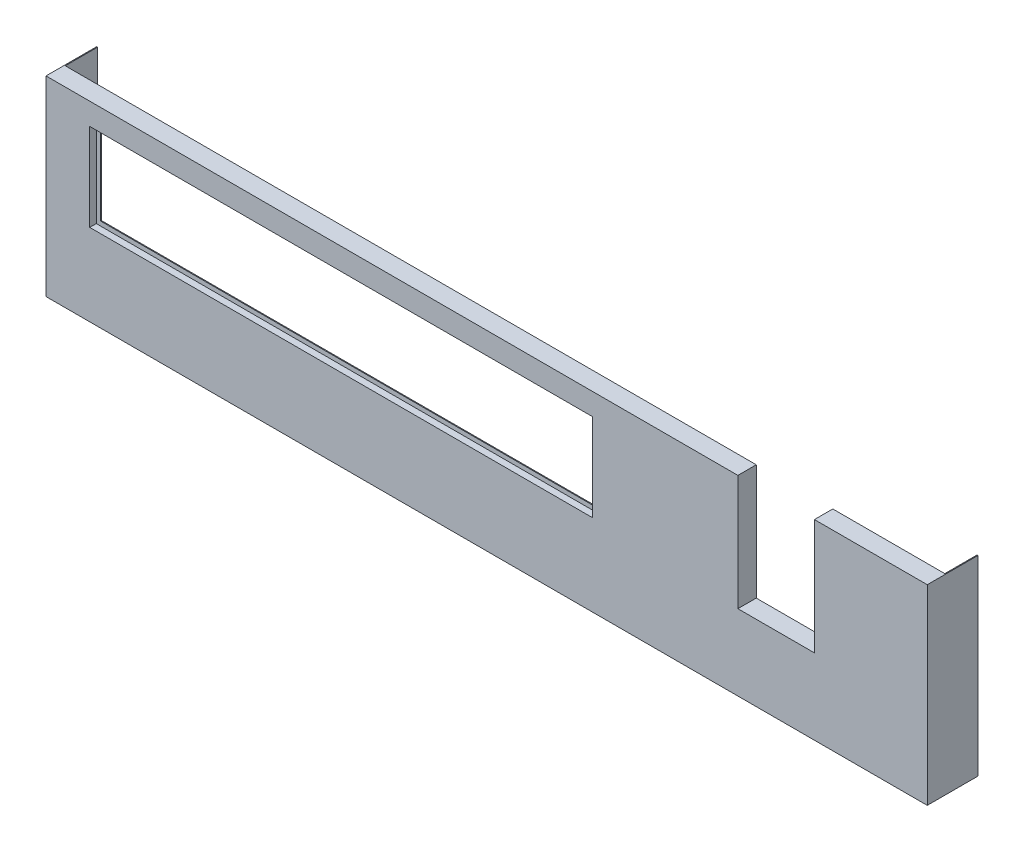
from build123d import *

# Parameters (mm, degrees)
EXTRUDE_1_DEPTH     = 2
SKETCH_7_W          = 2
SKETCH_7_H          = 437
EXTRUDE_2_DEPTH     = 114
SKETCH_8_W          = 2
SKETCH_8_H          = 437
EXTRUDE_3_DEPTH     = 114
EXTRUDE_4_DEPTH     = 40
SKETCH_10_W         = 1150
SKETCH_10_H         = 200
CUT_EXTRUDE_1_DEPTH = 10
SKETCH_11_W         = 2015
SKETCH_11_H         = 42.467862918
EXTRUDE_5_DEPTH     = 2
SKETCH_12_W         = 1154
SKETCH_12_H         = 204
SKETCH_12_W_2       = 1150
SKETCH_12_H_2       = 200
EXTRUDE_6_DEPTH     = 15
SKETCH_13_W         = 1154
SKETCH_13_H         = 204
SKETCH_13_W_2       = 1130
SKETCH_13_H_2       = 180
EXTRUDE_7_DEPTH     = 2


with BuildPart() as part:
    # 草图2 → 凸台-拉伸1 (new body)
    with BuildSketch(Plane.XY):
        Polygon((1757, 437), (2015, 437), (2015, 0), (0, 0), (0, 437), (1582, 437), (1582, 173), (1757, 173), align=None)
    extrude(amount=EXTRUDE_1_DEPTH)

    # 草图7 → 凸台-拉伸2 (add)
    with BuildSketch(Plane(origin=(0, 0, 0), x_dir=(-1, 0, 0), z_dir=(0, 0, -1))):
        with Locations((-2014, 218.5)):
            Rectangle(SKETCH_7_W, SKETCH_7_H)
    extrude(amount=EXTRUDE_2_DEPTH)

    # 草图8 → 凸台-拉伸3 (add)
    with BuildSketch(Plane(origin=(0, 0, 0), x_dir=(-1, 0, 0), z_dir=(0, 0, -1))):
        with Locations((-1, 218.5)):
            Rectangle(SKETCH_8_W, SKETCH_8_H)
    extrude(amount=EXTRUDE_3_DEPTH)

    # 草图9 → 凸台-拉伸4 (add)
    with BuildSketch(Plane(origin=(0, 0, 0), x_dir=(-1, 0, 0), z_dir=(0, 0, -1))):
        Polygon((-2013, 435), (-1759, 435), (-1759, 171), (-1580, 171), (-1580, 435), (-2, 435), (-2, 437), (-1582, 437), (-1582, 173), (-1757, 173), (-1757, 437), (-2013, 437), align=None)
    extrude(amount=EXTRUDE_4_DEPTH)

    # 草图10 → 切除-拉伸1 (cut)
    with BuildSketch(Plane.XY.offset(2)):
        with Locations((675, 287)):
            Rectangle(SKETCH_10_W, SKETCH_10_H)
    extrude(amount=-CUT_EXTRUDE_1_DEPTH, mode=Mode.SUBTRACT)

    # 草图11 → 凸台-拉伸5 (add)
    with BuildSketch(Plane.XZ):
        with Locations((1007.5, -19.233931459)):
            Rectangle(SKETCH_11_W, SKETCH_11_H)
    extrude(amount=-EXTRUDE_5_DEPTH)

    # 草图12 → 凸台-拉伸6 (add)
    with BuildSketch(Plane(origin=(0, 0, 0), x_dir=(-1, 0, 0), z_dir=(0, 0, -1))):
        with Locations((-675, 287)):
            Rectangle(SKETCH_12_W, SKETCH_12_H)
        with Locations((-675, 287)):
            Rectangle(SKETCH_12_W_2, SKETCH_12_H_2, mode=Mode.SUBTRACT)
    extrude(amount=EXTRUDE_6_DEPTH)

    # 草图13 → 凸台-拉伸7 (add)
    with BuildSketch(Plane(origin=(0, 0, -15), x_dir=(-1, 0, 0), z_dir=(0, 0, -1))):
        with Locations((-675, 287)):
            Rectangle(SKETCH_13_W, SKETCH_13_H)
        with Locations((-675, 287)):
            Rectangle(SKETCH_13_W_2, SKETCH_13_H_2, mode=Mode.SUBTRACT)
    extrude(amount=-EXTRUDE_7_DEPTH)


solid = part.part
